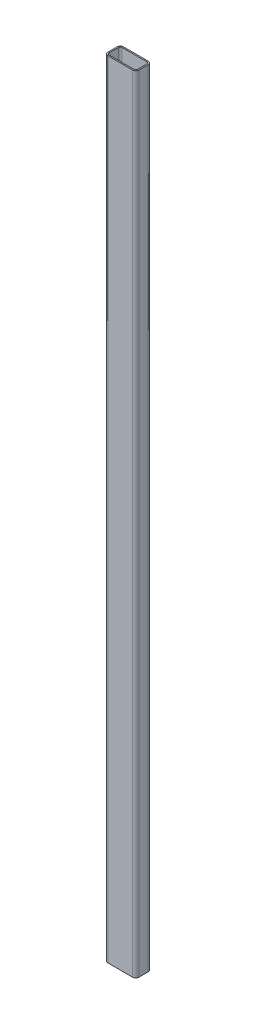
from build123d import *

# Parameters (mm, degrees)
EXTRUDE_THIN1_DEPTH = 1265


with BuildPart() as part:
    # Sketch1 → Extrude-Thin1 (new, symmetric)
    with BuildSketch(Plane(origin=(0, 0, 0), x_dir=(1, 0, 0), z_dir=(0, 1, 0))):
        with BuildLine():
            Line((-40, 25), (40, 25))
            ThreePointArc((40, 25), (47.071067812, 22.071067812), (50, 15))
            Line((50, 15), (50, -15))
            ThreePointArc((50, -15), (47.071067812, -22.071067812), (40, -25))
            Line((40, -25), (-40, -25))
            ThreePointArc((-40, -25), (-47.071067812, -22.071067812), (-50, -15))
            Line((-50, -15), (-50, 15))
            ThreePointArc((-50, 15), (-47.071067812, 22.071067812), (-40, 25))
        make_face()
        with BuildLine():
            Line((-40, 21), (40, 21))
            ThreePointArc((40, 21), (44.242640687, 19.242640687), (46, 15))
            Line((46, 15), (46, -15))
            ThreePointArc((46, -15), (44.242640687, -19.242640687), (40, -21))
            Line((40, -21), (-40, -21))
            ThreePointArc((-40, -21), (-44.242640687, -19.242640687), (-46, -15))
            Line((-46, -15), (-46, 15))
            ThreePointArc((-46, 15), (-44.242640687, 19.242640687), (-40, 21))
        make_face(mode=Mode.SUBTRACT)
    extrude(amount=EXTRUDE_THIN1_DEPTH, both=True)


solid = part.part
